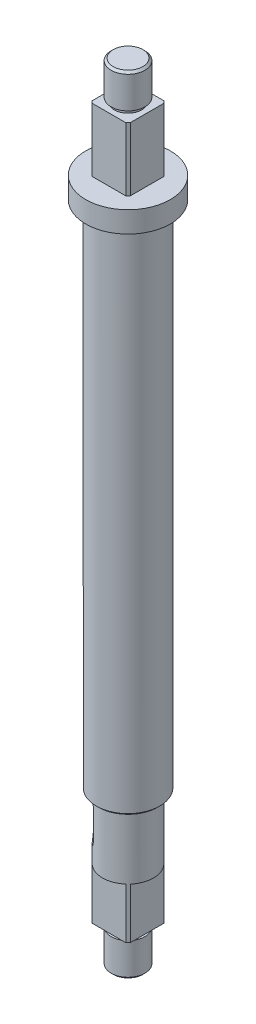
from build123d import *

# Parameters (mm, degrees)
SKETCH_2_OUTSIDE_W   = 117.256
SKETCH_2_OUTSIDE_H   = 117.256
SKETCH_2_OUTSIDE_W_2 = 18
SKETCH_2_OUTSIDE_H_2 = 18
CUT_EXTRUDE_1_DEPTH  = 30
SKETCH_3_OUTSIDE_W   = 117.256
SKETCH_3_OUTSIDE_H   = 117.256
SKETCH_3_OUTSIDE_W_2 = 18
SKETCH_3_OUTSIDE_H_2 = 18
CUT_EXTRUDE_2_DEPTH  = 24
CUT_EXTRUDE_START    = 8.5
CUT_EXTRUDE_3_DEPTH  = 24
CHAMFER_1_SIZE       = 1


with BuildPart() as part:
    # 草图1 → 旋转1 (revolve)
    with BuildSketch(Plane.XY, mode=Mode.PRIVATE) as revolve_1_sk:
        Polygon((0, -186), (0, 186), (-8, 186), (-8, 170), (-6.5, 170), (-6.5, 168), (-12, 168), (-12, 138), (-20, 138), (-20, 128), (-15, 128), (-15, -114), (-12, -114), (-12, -168), (-6.5, -168), (-6.5, -170), (-8, -170), (-8, -186), align=None)
    revolve(revolve_1_sk.sketch.rotate(Axis((0, -186, 0), (0, 1, 0)), 180), axis=Axis((0, -186, 0), (0, 1, 0)))

    # 草图2 outside → 切除-拉伸1 (cut)
    with BuildSketch(Plane(origin=(0, 168, 0), x_dir=(1, 0, 0), z_dir=(0, 1, 0))):
        Rectangle(SKETCH_2_OUTSIDE_W, SKETCH_2_OUTSIDE_H)
        Rectangle(SKETCH_2_OUTSIDE_W_2, SKETCH_2_OUTSIDE_H_2, mode=Mode.SUBTRACT)
    extrude(amount=-CUT_EXTRUDE_1_DEPTH, mode=Mode.SUBTRACT)

    # 草图3 outside → 切除-拉伸2 (cut)
    with BuildSketch(Plane.XZ.offset(168)):
        Rectangle(SKETCH_3_OUTSIDE_W, SKETCH_3_OUTSIDE_H)
        Rectangle(SKETCH_3_OUTSIDE_W_2, SKETCH_3_OUTSIDE_H_2, mode=Mode.SUBTRACT)
    extrude(amount=-CUT_EXTRUDE_2_DEPTH, mode=Mode.SUBTRACT)

    # 草图4 → 切除-拉伸3 (cut)
    with BuildSketch(Plane(origin=(0, 0, 0), x_dir=(0, -1, 0), z_dir=(-0.7071067811865488, 0, 0.7071067811865464)).offset(CUT_EXTRUDE_START)):
        with BuildLine():
            Line((119, 3), (133, 3))
            ThreePointArc((133, 3), (136, 0), (133, -3))
            Line((133, -3), (119, -3))
            ThreePointArc((119, -3), (116, 0), (119, 3))
        make_face()
    extrude(amount=CUT_EXTRUDE_3_DEPTH, mode=Mode.SUBTRACT)

    # 倒角1
    chamfer_1_edges = [part.edges().sort_by_distance(p)[0] for p in [
        (-8, -186, 0),
        (-15, -114, 0),
        (-8, 186, 0),
    ]]
    chamfer(chamfer_1_edges, length=CHAMFER_1_SIZE)


solid = part.part
